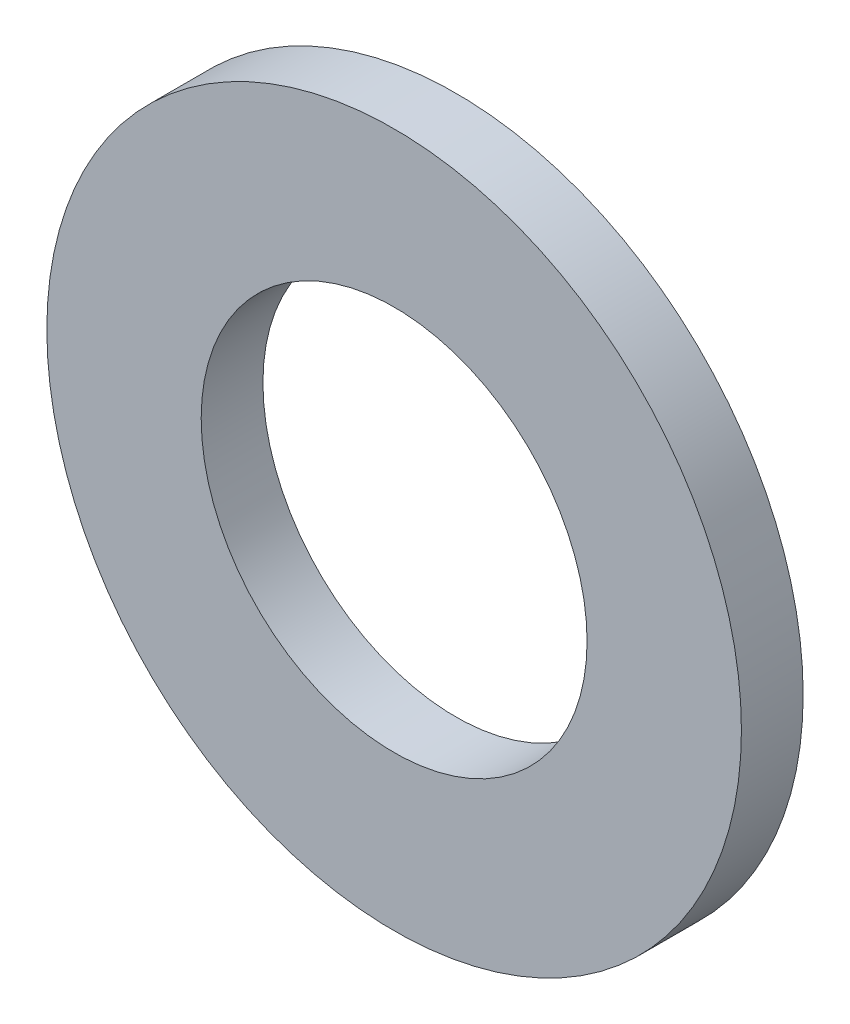
SolidWorks part; units mm, degrees
ref_plane "Front Plane" through (0, 0, 0) normal (0, 0, 1) x (1, 0, 0)
ref_plane "Top Plane" through (0, 0, 0) normal (0, 1, 0) x (1, 0, 0)
ref_plane "Right Plane" through (0, 0, 0) normal (1, 0, 0) x (0, 0, -1)
sketch "Sketch1" plane through (0, 0, 0) normal (0, 0, 1) x (1, 0, 0)
  circle A0 centre (0, 0) radius 45
  circle A1 centre (0, 0) radius 25
extrude "Boss-Extrude1" add sketch "Sketch1" along normal blind 8
sketch "Sketch2" plane through (0, 0, 8) normal (0, 0, 1) x (1, 0, 0)
  circle A0 centre (0, 0) radius 42
  circle A1 centre (0, 0) radius 25
extrude "Boss-Extrude2" add sketch "Sketch2" along normal blind 3
sketch "Sketch3" plane through (0, 0, 0) normal (0, 0, -1) x (-1, 0, 0)
  circle A1 centre (0, 37) radius 2.5
  circle A2 centre (32.0429, 18.5) radius 2.5
  circle A3 centre (32.0429, -18.5) radius 2.5
  circle A4 centre (0, -37) radius 2.5
  circle A5 centre (-32.0429, -18.5) radius 2.5
  circle A6 centre (-32.0429, 18.5) radius 2.5
  point P18 (0, 0)
  dimension "D1" = 6
extrude "Cut-Extrude1" cut sketch "Sketch3" against normal blind 6
chamfer "Chamfer1" distance 1 distance2 1 2 edges at (42, 0, 11) (25, 0, 11)
extrude "Cut-Extrude2" cut sketch "Sketch4" against normal blind 3
sketch "Sketch4" plane through (248.9939, -65.3327, 8) normal (0, 0, -1) x (0.8405, -0.5418, 0)
  circle A0 centre (-244.676, 80) radius 42
  circle A1 centre (-244.676, -130) radius 55
